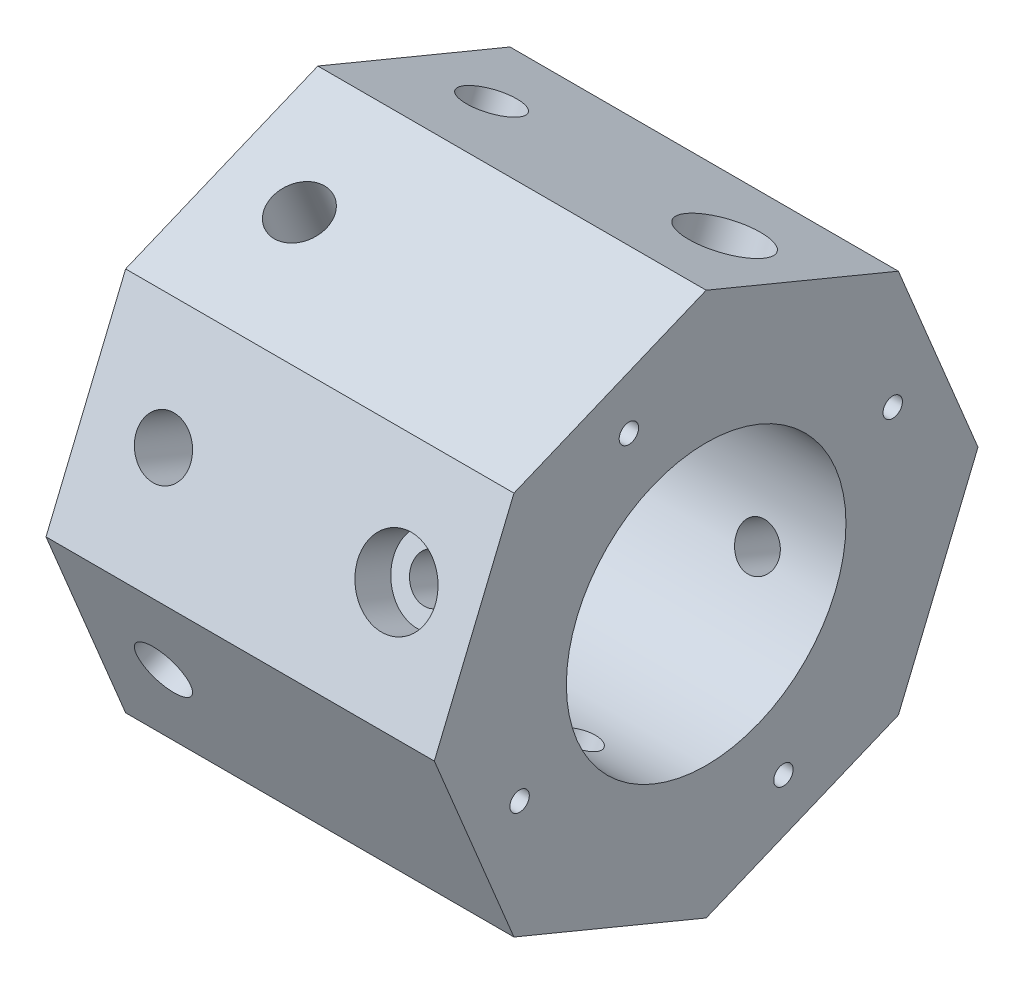
SolidWorks part; units mm, degrees
ref_plane "前视基准面" through (0, 0, 0) normal (0, 0, 1) x (1, 0, 0)
ref_plane "上视基准面" through (0, 0, 0) normal (0, 1, 0) x (1, 0, 0)
ref_plane "右视基准面" through (0, 0, 0) normal (1, 0, 0) x (0, 0, -1)
sketch "草图1" plane through (0, 0, 0) normal (1, 0, 0) x (0, 0, -1)
  line L0 (24.7487, 24.7487) -> (0, 35)
  line L1 (-24.7487, 24.7487) -> (-35, 0)
  line L2 (-35, 0) -> (-24.7487, -24.7487)
  line L3 (-24.7487, -24.7487) -> (0, -35)
  line L4 (0, -35) -> (24.7487, -24.7487)
  line L5 (24.7487, -24.7487) -> (35, 0)
  line L6 (35, 0) -> (24.7487, 24.7487)
  line L7 (0, 35) -> (-24.7487, 24.7487)
  circle A0 centre (0, 0) radius 18
  circle A1 centre (0, 0) radius 35
  circle A2 centre (0, 0) radius 32.3358 construction
  dimension "D1" = 36
  dimension "D2" = 70
extrude "凸台-拉伸1" add sketch "草图1" along normal mid plane 50 contours L0 L7 L1 L2 L3 L4 L5 L6 A0
sketch "草图2" plane through (0, -29.8744, 12.3744) normal (0, 0.9239, -0.3827) x (1, 0, 0)
  line L0 (15, 0) -> (25, 0) construction
  line L1 (25, -32.3358) -> (25, -13.3939) construction
  line L2 (25, -13.3939) -> (25, 13.3939) construction
  circle A0 centre (15, 0) radius 5
  dimension "D1" = 10
  dimension "D2" = 10
extrude "切除-拉伸1" cut sketch "草图2" along normal blind 5
sketch "草图4" plane through (0, -25.255, 10.461) normal (0, -0.9239, 0.3827) x (1, 0, 0)
  circle A0 centre (15, 0) radius 2.75
  dimension "D1" = 5.5
extrude "切除-拉伸2" cut sketch "草图4" against normal blind 23
sketch "草图5" plane through (0, -12.3744, 29.8744) normal (0, -0.3827, 0.9239) x (1, 0, 0)
  line L0 (-25, 0) -> (-15, 0) construction
  line L1 (-25, 13.3939) -> (-25, -13.3939) construction
  dimension "D1" = 10
hole_wizard "M8x1.0 螺纹孔1" positions "3D草图2" profile "草图6" tap size "M8x1.0" standard "BSI"
sketch3d "3D草图2"
  point P0 (-15, -12.3744, 29.8744)
sketch "草图6" plane through (-15, -12.3744, 29.8744) normal (1, 0, 0) x (0, -0.9239, -0.3827)
  line L0 (0, 0) -> (0, 17.103)
  line L1 (0, 17.103) -> (3.5, 15)
  line L2 (3.5, 15) -> (3.5, 0)
  line L5 (3.5, 0) -> (0, 0)
  line L10 (0, 17.103) -> (-3.5, 15) construction
  line L11 (0, -6.35) -> (0, 107.95) construction
  dimension "螺纹孔钻头直径" = 7
  dimension "螺纹孔钻头深度" = 15
  dimension "导头角度" = 118
cosmetic thread "孔螺蚊线1" parameters "D1"=10, "D2"=8
pattern_circular "阵列(圆周)1" count 8 over 360 about axis through (25, 0, 0) along (-1, 0, 0) of "M8x1.0 螺纹孔1"
cosmetic thread "孔螺蚊线2" parameters "D1"=10, "D2"=8
cosmetic thread "孔螺蚊线3" parameters "D1"=10, "D2"=8
cosmetic thread "孔螺蚊线4" parameters "D1"=10, "D2"=8
cosmetic thread "孔螺蚊线5" parameters "D1"=10, "D2"=8
cosmetic thread "孔螺蚊线6" parameters "D1"=10, "D2"=8
cosmetic thread "孔螺蚊线7" parameters "D1"=10, "D2"=8
cosmetic thread "孔螺蚊线8" parameters "D1"=10, "D2"=8
pattern_circular "阵列(圆周)2" count 4 over 360 about axis through (0, 0, 0) along (1, 0, 0) of "切除-拉伸1", "切除-拉伸2"
sketch "草图7" plane through (25, 0, 0) normal (1, 0, 0) x (0, 0, -1)
  line L0 (0, 0) -> (24.0209, 9.9498) construction
  line L1 (24.0209, 9.9498) -> (29.8744, 12.3744) construction
  line L2 (35, 0) -> (24.7487, 24.7487) construction
  dimension "D1" = 26
hole_wizard "M3x0.5 螺纹孔1" positions "3D草图3" profile "草图8" tap size "M3x0.5" standard "BSI"
sketch3d "3D草图3"
  point P0 (25, 9.9498, -24.0209)
sketch "草图8" plane through (25, 9.9498, -24.0209) normal (0, 1, 0) x (0, 0, -1)
  line L0 (0, 0) -> (0, 8.2511)
  line L1 (0, 8.2511) -> (1.25, 7.5)
  line L2 (1.25, 7.5) -> (1.25, 0)
  line L5 (1.25, 0) -> (0, 0)
  line L10 (0, 8.2511) -> (-1.25, 7.5) construction
  line L11 (0, -6.35) -> (0, 107.95) construction
  dimension "螺纹孔钻头直径" = 2.5
  dimension "螺纹孔钻头深度" = 7.5
  dimension "导头角度" = 118
cosmetic thread "孔螺蚊线9" parameters "D1"=6, "D2"=3
pattern_circular "阵列(圆周)3" count 4 over 360 about axis through (0, 0, 0) along (1, 0, 0) of "M3x0.5 螺纹孔1"
cosmetic thread "孔螺蚊线10" parameters "D1"=6, "D2"=3
cosmetic thread "孔螺蚊线11" parameters "D1"=6, "D2"=3
cosmetic thread "孔螺蚊线12" parameters "D1"=6, "D2"=3
